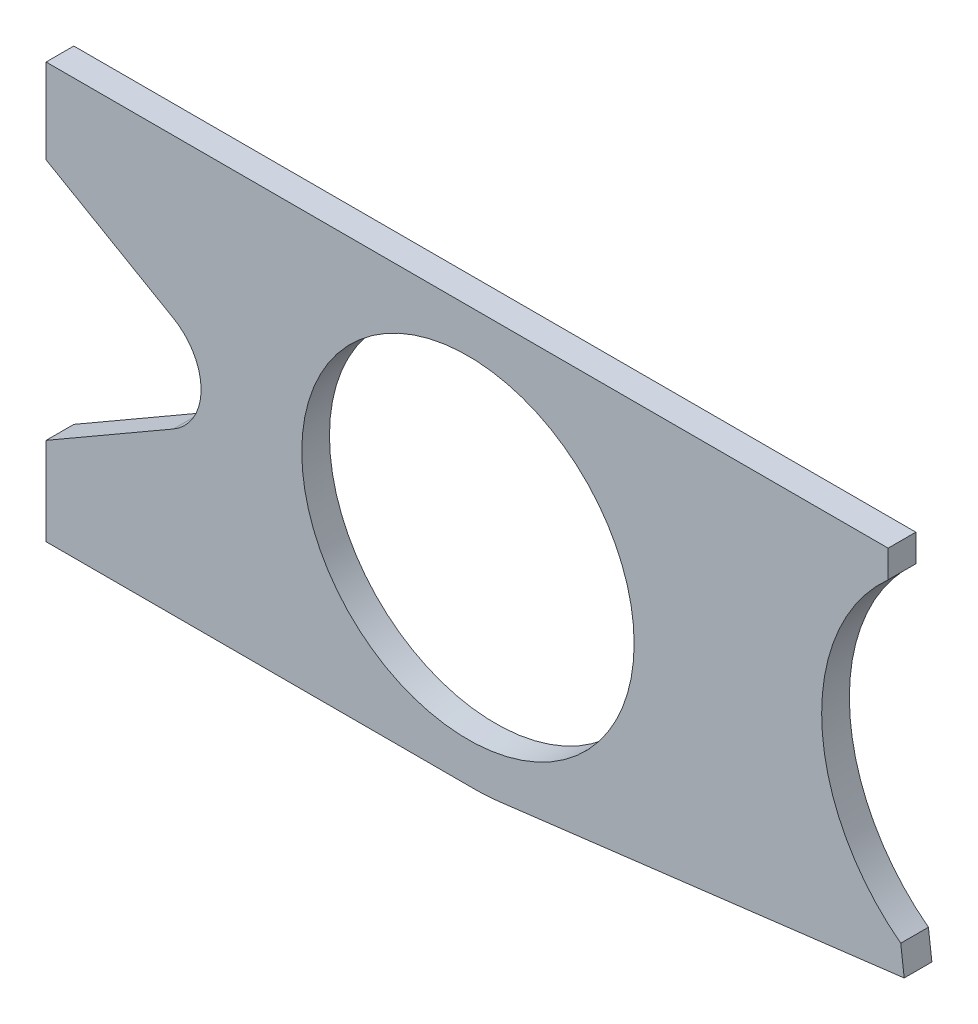
SolidWorks part; units mm, degrees
ref_plane "Front Plane" through (0, 0, 0) normal (0, 0, 1) x (1, 0, 0)
ref_plane "Top Plane" through (0, 0, 0) normal (0, 1, 0) x (1, 0, 0)
ref_plane "Right Plane" through (0, 0, 0) normal (1, 0, 0) x (0, 0, -1)
sketch "Sketch1" plane through (0, 0, 0) normal (0, 0, 1) x (1, 0, 0)
  line L0 (-42.2835, 0) -> (36.9087, 0) construction
  line L1 (0, 40.0297) -> (0, -42.6309) construction
  line L2 (-48.3, 63.7) -> (-48.3, 53.7996)
  line L3 (-48.3, 63.7) -> (-352.3, 63.7)
  line L4 (-352.3, 63.7) -> (-352.3, 33.1)
  line L5 (-352.3, 33.1) -> (-306.3496, 6.5705)
  line L6 (-306.3496, -28.0705) -> (-352.3, -54.6)
  line L7 (-352.3, -54.6) -> (-352.3, -86.3)
  line L8 (-352.3, -86.3) -> (-197.7576, -86.3)
  line L9 (-188.6174, -85.741) -> (-42.5, -67.8)
  line L10 (-42.5, -67.8) -> (-43.758, -57.5546)
  line L11 (-352.3, 33.1) -> (-352.3, -54.6) construction
  line L12 (-352.3, -10.75) -> (-222.9308, -10.75) construction
  line L13 (-42.5, -35.2985) -> (-42.5, -67.8) construction
  line L14 (-200, 48.881) -> (-200, -145.578) construction
  line L15 (-185.4437, -12) -> (-281.2544, -12) construction
  arc A0 (-48.3, 53.7996) -> (-43.758, -57.5546) centre (0, 0) ccw
  arc A1 (-306.3496, -28.0705) -> (-306.3496, 6.5705) centre (-316.3496, -10.75) ccw
  arc A2 (-188.6174, -85.741) -> (-197.7576, -86.3) centre (-197.7576, -11.3) cw
  circle A3 centre (-200, -12) radius 60
  point P22 (-276.3496, -10.75)
  dimension "D1" = 144.6
  dimension "D9" = 20
  dimension "D13" = 75
  dimension "D16" = 120
  dimension "D2" = 48.3
  dimension "D3" = 63.7
  dimension "D4" = 352.3
  dimension "D5" = 30.6
  dimension "D6" = 150
  dimension "D7" = 31.7
  dimension "D8" = 60
  dimension "D10" = 173
  dimension "D11" = 42.5
  dimension "D12" = 67.8
  dimension "D14" = 200
  dimension "D15" = 12
extrude "Boss-Extrude1" add sketch "Sketch1" along normal blind 10
